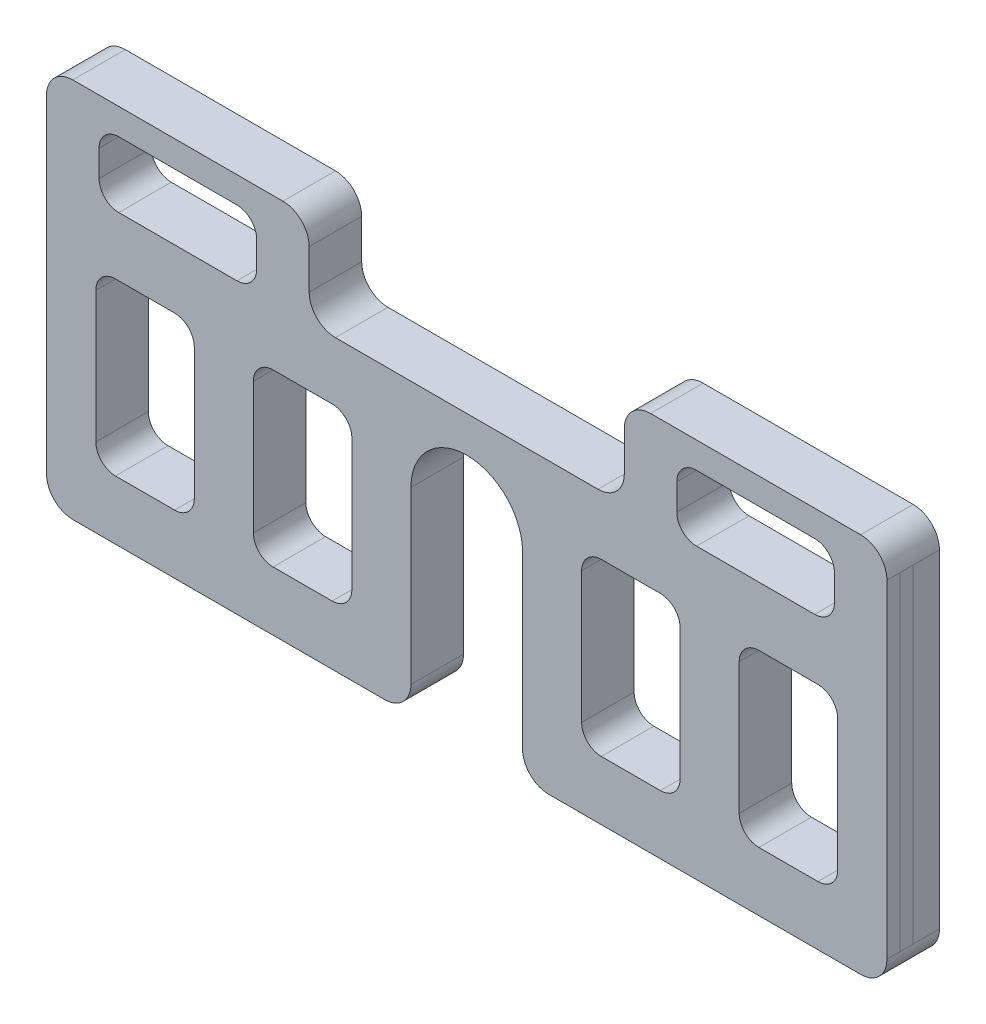
from build123d import *

# Parameters (mm, degrees)
SKETCH1_W            = 120
SKETCH1_H            = 50
BOSS_EXTRUDE1_DEPTH  = 20
FILLET1_R            = 15
SKETCH2_W            = 75
SKETCH2_H            = 130
CUT_EXTRUDE1_DEPTH   = 433.319326424
FILLET2_R            = 15
FILLET2_OF_MIRROR1_R = 15


with BuildPart() as part:
    # Sketch1 → Boss-Extrude1 (new, symmetric)
    with BuildSketch(Plane.XY):
        with BuildLine():
            Line((42.5, 150), (42.5, 20))
            ThreePointArc((42.5, 20), (48.357864376, 5.857864376), (62.5, 0))
            Line((62.5, 0), (300, 0))
            ThreePointArc((300, 0), (314.142135624, 5.857864376), (320, 20))
            Line((320, 20), (320, 270))
            ThreePointArc((320, 270), (314.142135624, 284.142135624), (300, 290))
            Line((300, 290), (140, 290))
            ThreePointArc((140, 290), (125.857864376, 284.142135624), (120, 270))
            Line((120, 270), (120, 240))
            ThreePointArc((120, 240), (114.142135624, 225.857864376), (100, 220))
            Line((100, 220), (-100, 220))
            ThreePointArc((-100, 220), (-114.142135624, 225.857864376), (-120, 240))
            Line((-120, 240), (-120, 270))
            ThreePointArc((-120, 270), (-125.857864376, 284.142135624), (-140, 290))
            Line((-140, 290), (-300, 290))
            ThreePointArc((-300, 290), (-314.142135624, 284.142135624), (-320, 270))
            Line((-320, 270), (-320, 20))
            ThreePointArc((-320, 20), (-314.142135624, 5.857864376), (-300, 0))
            Line((-300, 0), (-62.5, 0))
            ThreePointArc((-62.5, 0), (-48.357864376, 5.857864376), (-42.5, 20))
            Line((-42.5, 20), (-42.5, 150))
            ThreePointArc((-42.5, 150), (0, 192.5), (42.5, 150))
        make_face()
        with Locations((-220, 245)):
            Rectangle(SKETCH1_W, SKETCH1_H, mode=Mode.SUBTRACT)
        with Locations((220, 245)):
            Rectangle(SKETCH1_W, SKETCH1_H, mode=Mode.SUBTRACT)
    extrude(amount=BOSS_EXTRUDE1_DEPTH, both=True)

    # Fillet1
    fillet1_edges = [part.edges().sort_by_distance(p)[0] for p in [
        (-160, 220, 0),
        (-160, 270, 0),
        (-280, 270, 0),
        (-280, 220, 0),
        (280, 220, 0),
        (280, 270, 0),
        (160, 270, 0),
        (160, 220, 0),
    ]]
    fillet(fillet1_edges, radius=FILLET1_R)

    # Sketch2 → Cut-Extrude1 (cut, symmetric)
    with BuildSketch(Plane.XY):
        with Locations((-245, 110)):
            Rectangle(SKETCH2_W, SKETCH2_H)
        with Locations((-125, 110)):
            Rectangle(SKETCH2_W, SKETCH2_H)
    cut_extrude1 = extrude(amount=CUT_EXTRUDE1_DEPTH, both=True, mode=Mode.SUBTRACT)

    # Fillet2
    fillet2_edges = [part.edges().sort_by_distance(p)[0] for p in [
        (-207.5, 175, 0),
        (-207.5, 45, 0),
        (-282.5, 45, 0),
        (-282.5, 175, 0),
        (-87.5, 175, 0),
        (-87.5, 45, 0),
        (-162.5, 45, 0),
        (-162.5, 175, 0),
    ]]
    fillet(fillet2_edges, radius=FILLET2_R)

    # Mirror1: Cut-Extrude1 across plane
    add(cut_extrude1.mirror(Plane(origin=(0, 0, 0), x_dir=(0, 0, 1), z_dir=(1, 0, 0))), mode=Mode.SUBTRACT)

    # Fillet2 of Mirror1
    fillet2_of_mirror1_edges = [part.edges().sort_by_distance(p)[0] for p in [
        (207.5, 175, 0),
        (207.5, 45, 0),
        (282.5, 45, 0),
        (282.5, 175, 0),
        (87.5, 175, 0),
        (87.5, 45, 0),
        (162.5, 45, 0),
        (162.5, 175, 0),
    ]]
    fillet(fillet2_of_mirror1_edges, radius=FILLET2_OF_MIRROR1_R)


solid = part.part
